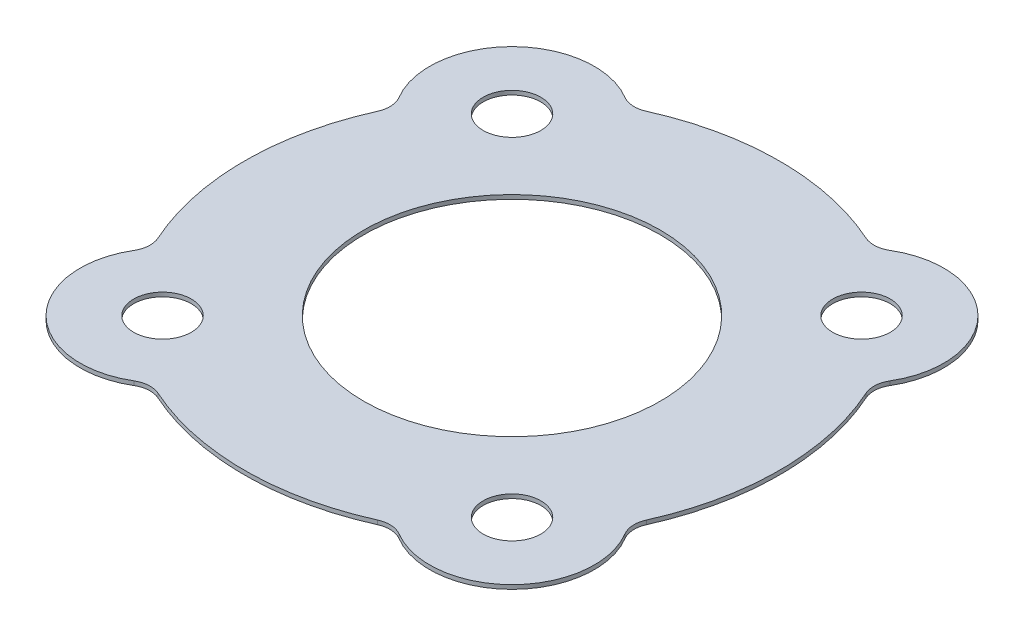
SolidWorks part; units mm, degrees
ref_plane "Front Plane" through (0, 0, 0) normal (0, 0, 1) x (1, 0, 0)
ref_plane "Top Plane" through (0, 0, 0) normal (0, 1, 0) x (1, 0, 0)
ref_plane "Right Plane" through (0, 0, 0) normal (1, 0, 0) x (0, 0, -1)
other "Configuration Table"
sketch "Sketch1" plane through (0, 0, 0) normal (0, 1, 0) x (1, 0, 0)
  line L0 (0, 72.7288) -> (0, 0) construction
  line L1 (0, 0) -> (-83.6381, 0) construction
  line L2 (0, 0) -> (-54.181, 54.181) construction
  circle A0 centre (0, 0) radius 32.5
  circle A1 centre (0, 0) radius 30 construction
  circle A2 centre (-21.2132, 21.2132) radius 10
  circle A3 centre (21.2132, 21.2132) radius 10
  circle A4 centre (21.2132, -21.2132) radius 10
  circle A5 centre (-21.2132, -21.2132) radius 10
  point P18 (0, 0)
  dimension "D1" = 65
  dimension "D2" = 60
  dimension "D4" = 20
  dimension "D3" = 45
  dimension "D5" = 4
extrude "Boss-Extrude1" add sketch "Sketch1" along normal blind 0.5 contours A5 A0 A4 A3 A2 | A0 A2 | A0 A2 | A0 A3 | A0 A3 | A0 A4 | A0 A4 | A0 A5 | A0 A5
sketch "Sketch2" plane through (0, 0.5, 0) normal (0, 1, 0) x (1, 0, 0)
  circle A0 centre (0, 0) radius 18
  circle A1 centre (0, 0) radius 30 construction
  circle A2 centre (21.2132, 21.2132) radius 3.5
  circle A3 centre (21.2132, -21.2132) radius 3.5
  circle A4 centre (-21.2132, -21.2132) radius 3.5
  circle A5 centre (-21.2132, 21.2132) radius 3.5
  point P15 (0, 0)
  dimension "D1" = 60
  dimension "D2" = 36
  dimension "D3" = 7
  dimension "D4" = 4
extrude "Cut-Extrude1" cut sketch "Sketch2" against normal blind 50
fillet "Fillet1" radius 3 8 edges at (28.916, 0.25, 14.8362) (14.8362, 0.25, 28.916) (-28.916, 0.25, -14.8362) (-14.8362, 0.25, -28.916) (-14.8362, 0.25, 28.916) (-28.916, 0.25, 14.8362) (14.8362, 0.25, -28.916) (28.916, 0.25, -14.8362)
